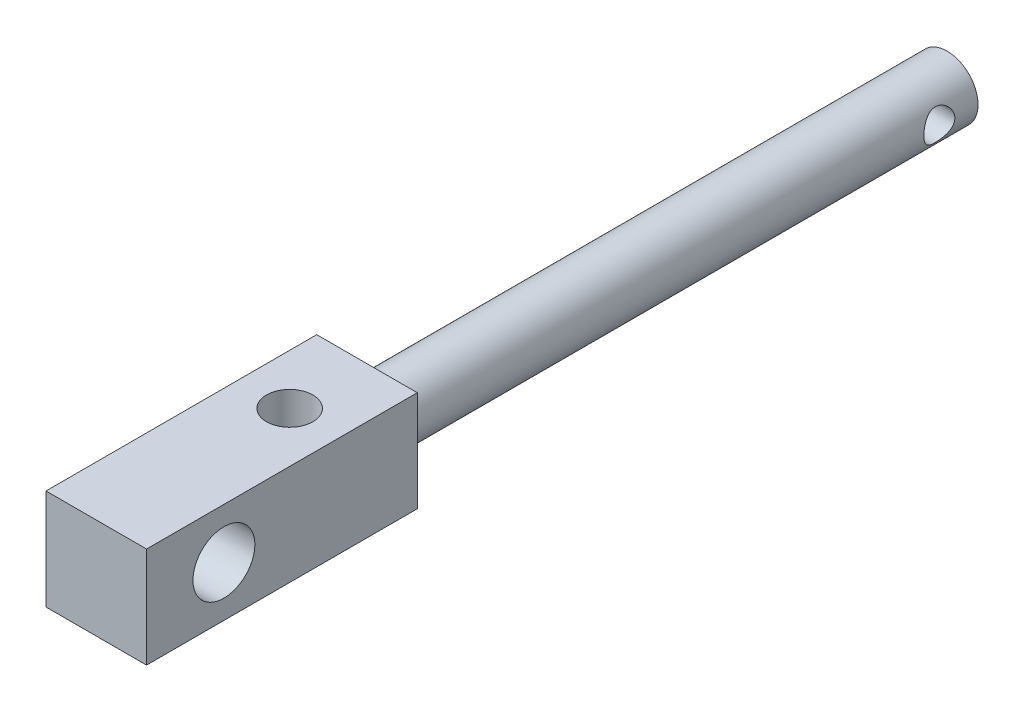
SolidWorks part; units mm, degrees
ref_plane "前视基准面" through (0, 0, 0) normal (0, 0, 1) x (1, 0, 0)
ref_plane "上视基准面" through (0, 0, 0) normal (0, 1, 0) x (1, 0, 0)
ref_plane "右视基准面" through (0, 0, 0) normal (1, 0, 0) x (0, 0, -1)
sketch "草图1" plane through (0, 0, 0) normal (0, 0, 1) x (1, 0, 0)
  line L1 (6.5, -6.5) -> (-6.5, -6.5)
  line L2 (6.5, -6.5) -> (6.5, 6.5)
  line L3 (6.5, 6.5) -> (-6.5, 6.5)
  line L4 (-6.5, -6.5) -> (-6.5, 6.5)
  line L5 (6.5, -6.5) -> (-6.5, 6.5) construction
  line L6 (6.5, 6.5) -> (-6.5, -6.5) construction
  point P0 (0, 0)
  dimension "D1" = 13
extrude "凸台-拉伸1" add sketch "草图1" along normal mid plane 20
sketch "草图3" plane through (0, 6.5, 0) normal (0, 1, 0) x (1, 0, 0)
  circle A0 centre (0, 0) radius 3
  dimension "D1" = 6
extrude "切除-拉伸1" cut sketch "草图3" against normal blind 20
sketch "草图4" plane through (0, 0, -10) normal (0, 0, -1) x (-1, 0, 0)
  circle A0 centre (0, 0) radius 4
  dimension "D1" = 8
extrude "凸台-拉伸2" add sketch "草图4" along normal blind 75
sketch "草图5" plane through (0, 0, 10) normal (0, 0, 1) x (1, 0, 0)
  line L4 (-6.5, 6.5) -> (-6.5, -6.5)
  line L5 (-6.5, -6.5) -> (6.5, -6.5)
  line L6 (6.5, -6.5) -> (6.5, 6.5)
  line L7 (6.5, 6.5) -> (-6.5, 6.5)
  line L8 (-6.5, 6.5) -> (-6.5, -6.5)
  line L9 (-6.5, -6.5) -> (6.5, -6.5)
  line L10 (6.5, -6.5) -> (6.5, 6.5)
  line L11 (6.5, 6.5) -> (-6.5, 6.5)
  dimension "D1" = 0
extrude "凸台-拉伸3" add sketch "草图5" along normal blind 15
sketch "草图6" plane through (-6.5, 0, 0) normal (-1, 0, 0) x (0, 0, 1)
  line L0 (15, 0) -> (25, 0) construction
  line L1 (25, 6.5) -> (25, -6.5) construction
  circle A0 centre (15, 0) radius 4
  dimension "D1" = 10
  dimension "D2" = 8
extrude "切除-拉伸2" cut sketch "草图6" against normal blind 37
sketch "草图7" plane through (-6.5, 0, 0) normal (-1, 0, 0) x (0, 0, 1)
  line L0 (-80, 4) -> (-80, 0) construction
  line L1 (-10, 4) -> (-85, 4) construction
  line L2 (-80, 0) -> (-80, -4) construction
  line L3 (-85, -4) -> (-10, -4) construction
  line L4 (-85, 4) -> (-85, -4) construction
  circle A0 centre (-80, 0) radius 2
  dimension "D1" = 4
  dimension "D2" = 5
extrude "切除-拉伸3" cut sketch "草图7" against normal blind 300
